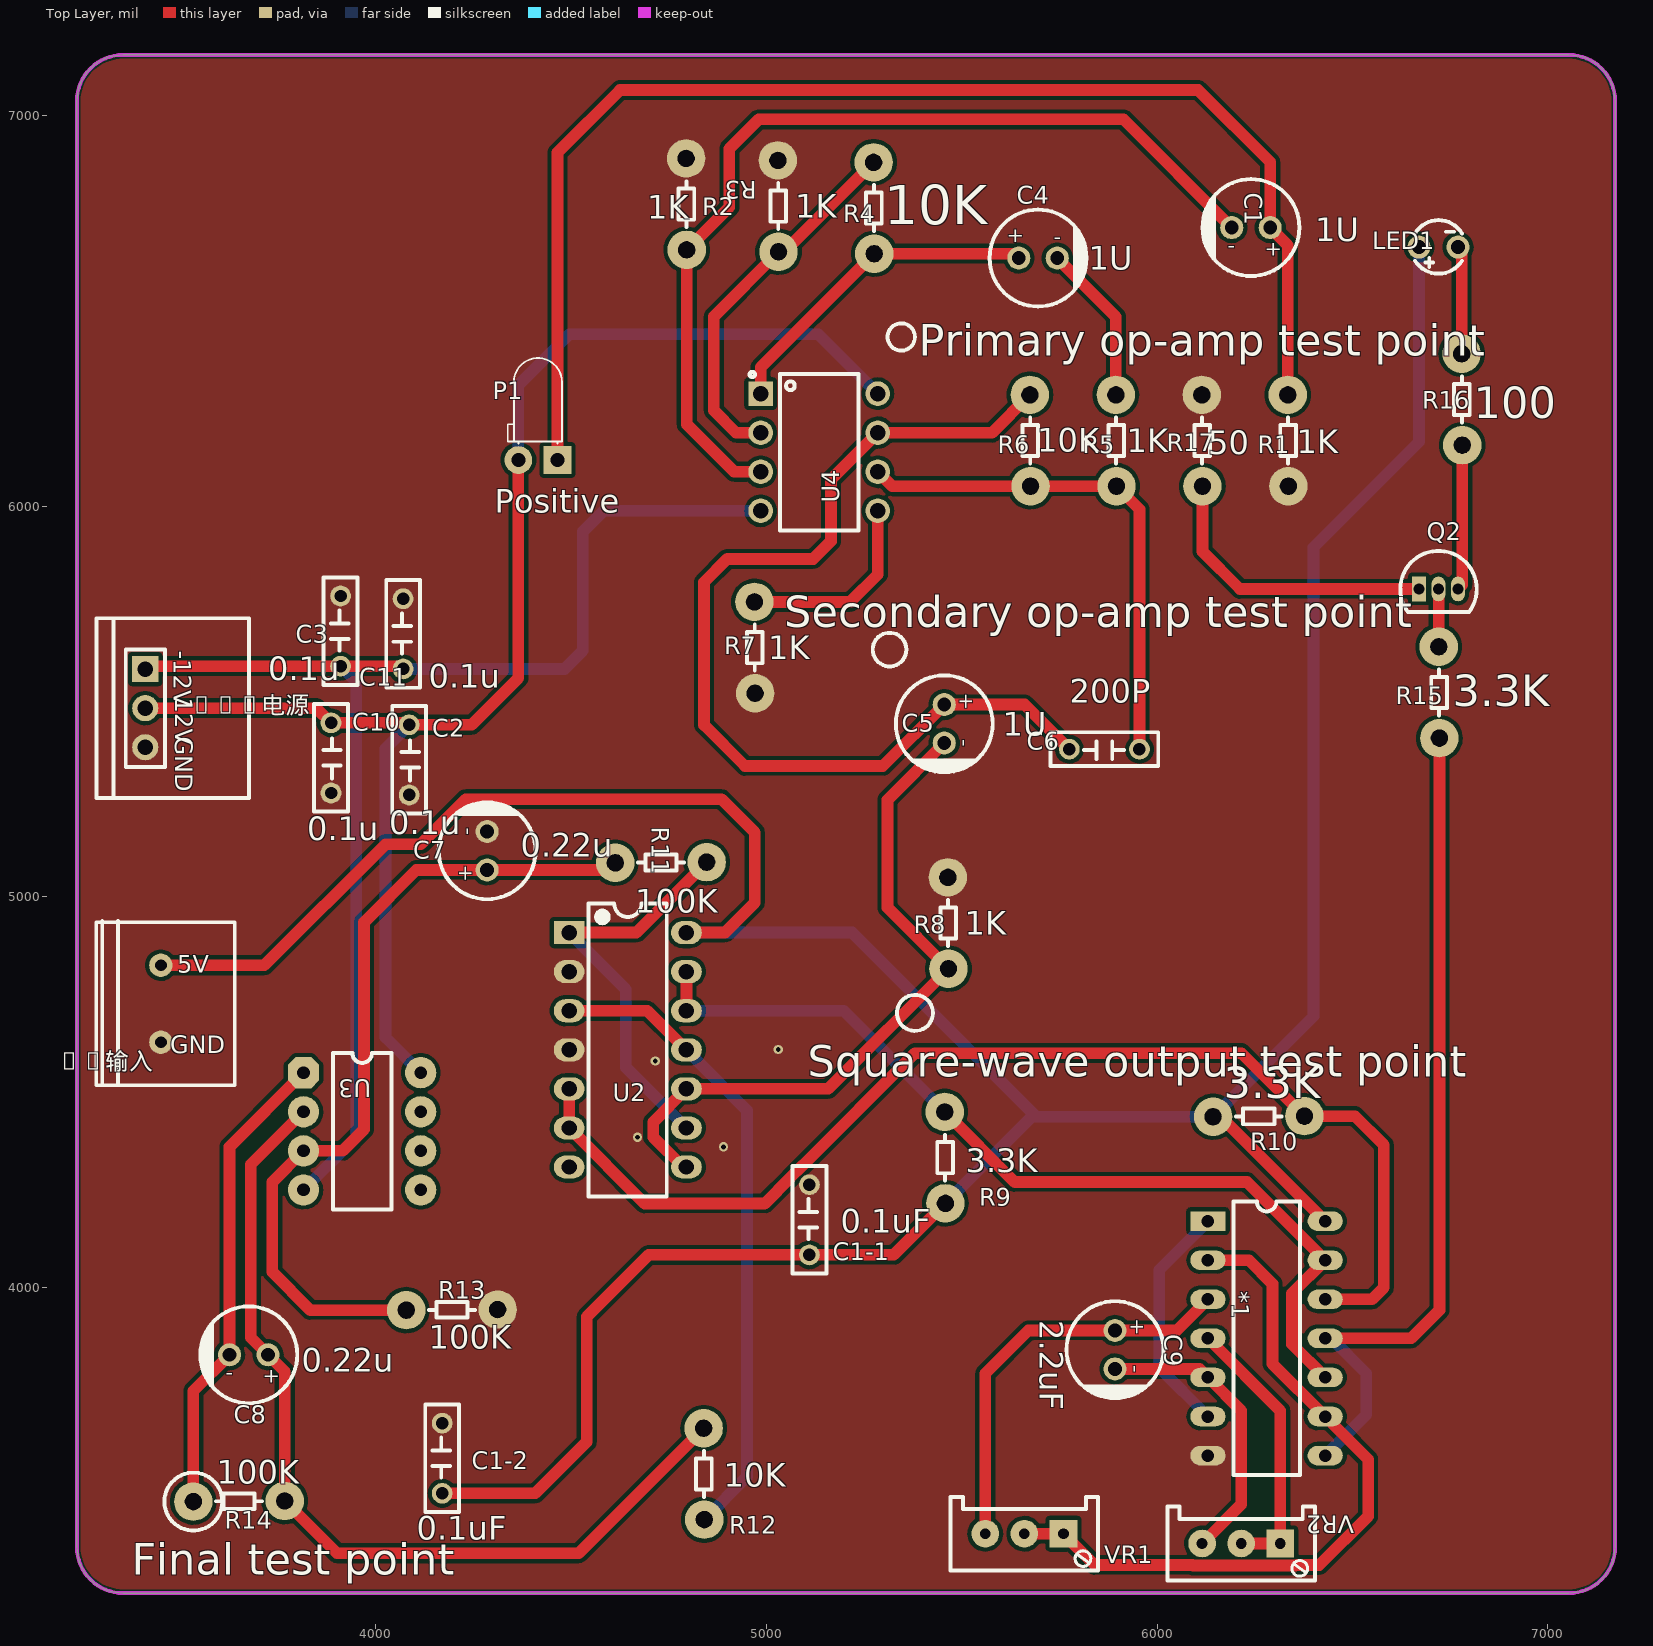
[diagram p0: Top Layer view]
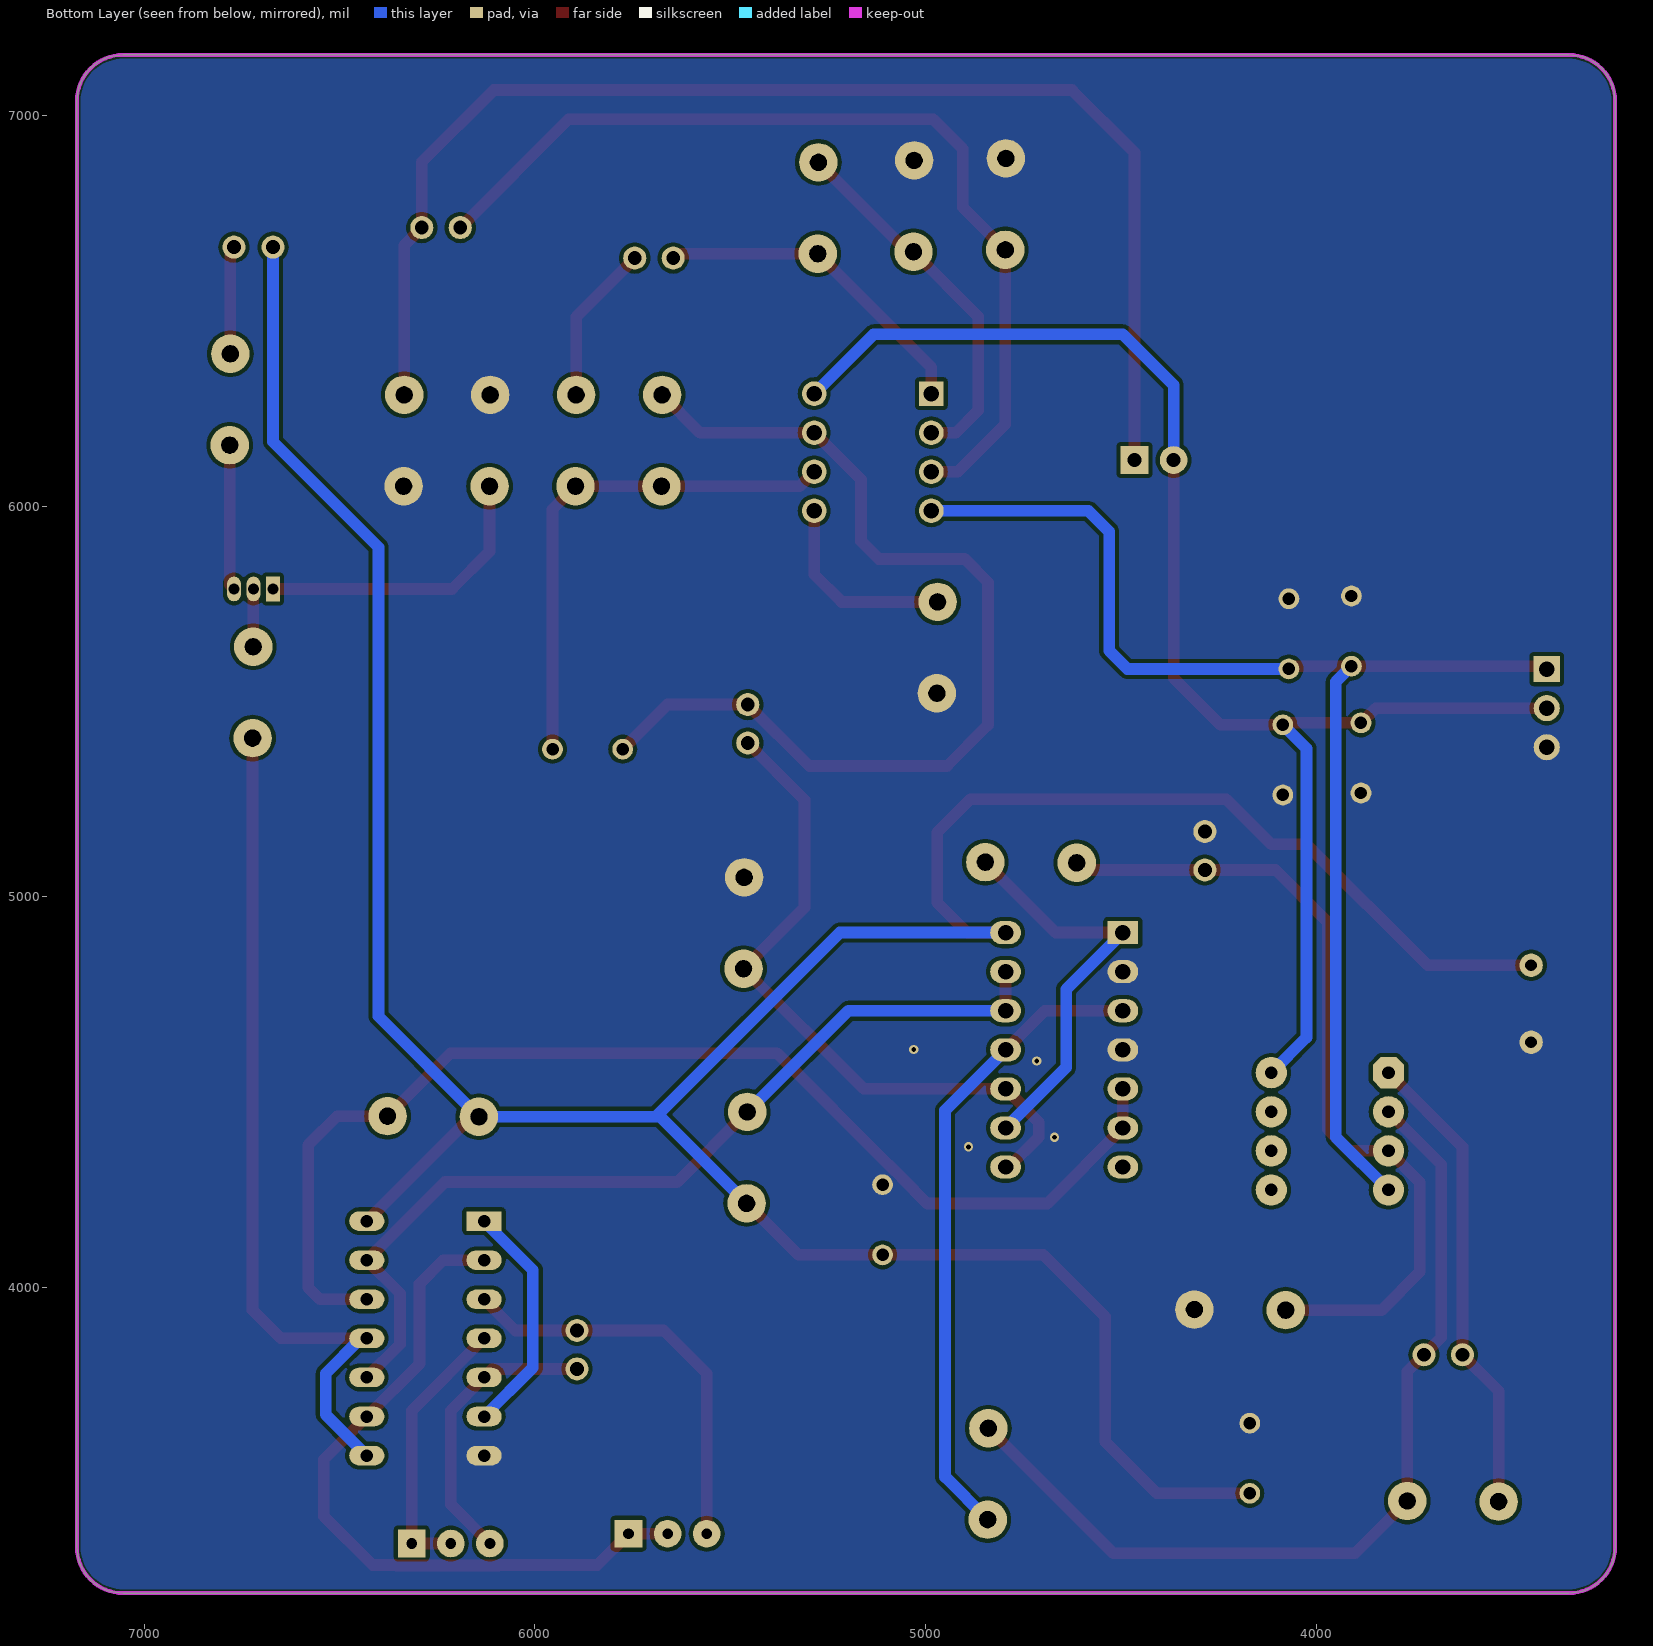
[diagram p1: Bottom Layer view, seen from below]
# Altium PCB MISC75397.pcbdoc
Units mil, origin at the board's own origin, x right, y up, seen from the top; angles counter-clockwise.
Board outline 3937.01 x 3937.01 mil, 2 copper layers (Top Layer, Bottom Layer), stack 62.206 mil thick; 41 components, 30 nets, 122 pads, 4 vias.

## Layer stack, top to bottom
Top Solder Mask Layer: solder mask 0.394, Dk 3.3
Top Layer: signal copper 1.379
Dielectric1: surface 59.449, FR4, Dk 4.5
Bottom Layer: signal copper 1.378
Bottom Solder Mask Layer: solder mask 0.394, Dk 3.3

## Board outline
3235,3336.1 ccw(c3353.11,3336.1) 3353.11,3217.99 7053.9,3217.99 ccw(c7053.9,3336.1) 7172.01,3336.1 7172.01,7036.89 ccw(c7053.9,7036.89) 7053.9,7155 3353.11,7155 ccw(c3353.11,7036.89) 3235,7036.89

## Design rules (kind name [scope] priority, off if disabled: settings)
BoardOutlineClearance copperThickness2oz_1 [All] p2 off: genericclearance=7.99 ignorepadtopadclearanceinfootprint=FALSE except(0: Arc-SplitContinuation Track-SplitContinuation SMDPad-SplitContinuation THPad-SplitContinuation Via-SplitContinuation Fill-SplitContinuation Region-SplitContinuation Poly-SplitContinuation Text-SplitContinuation Hole-SplitContinuation; 5.98: Arc-CutoutEdge Track-CutoutEdge SMDPad-CutoutEdge THPad-CutoutEdge Via-CutoutEdge Text-CutoutEdge; 6.89: Hole-OutlineEdge Hole-CutoutEdge; 10: Poly-OutlineEdge Poly-CutoutEdge; 11.81: Arc-OutlineEdge Track-OutlineEdge SMDPad-OutlineEdge THPad-OutlineEdge Via-OutlineEdge Fill-OutlineEdge Region-OutlineEdge Text-OutlineEdge Fill-CutoutEdge Region-CutoutEdge)
BoardOutlineClearance Plane_innerPlane_1 [All] p4 off: genericclearance=4.02 ignorepadtopadclearanceinfootprint=FALSE except(0: Arc-SplitContinuation Track-SplitContinuation SMDPad-SplitContinuation THPad-SplitContinuation Via-SplitContinuation Fill-SplitContinuation Region-SplitContinuation Poly-SplitContinuation Text-SplitContinuation Hole-SplitContinuation; 5.98: Arc-CutoutEdge Track-CutoutEdge SMDPad-CutoutEdge THPad-CutoutEdge Via-CutoutEdge Text-CutoutEdge; 6.89: Hole-OutlineEdge Hole-CutoutEdge; 10: Poly-OutlineEdge Poly-CutoutEdge; 11.81: Arc-OutlineEdge Track-OutlineEdge SMDPad-OutlineEdge THPad-OutlineEdge Via-OutlineEdge Fill-OutlineEdge Region-OutlineEdge Text-OutlineEdge Fill-CutoutEdge Region-CutoutEdge)
BoardOutlineClearance Copper_copperRegion_1 [All] p6 off: genericclearance=4.02 ignorepadtopadclearanceinfootprint=FALSE except(0: Arc-SplitContinuation Track-SplitContinuation SMDPad-SplitContinuation THPad-SplitContinuation Via-SplitContinuation Fill-SplitContinuation Region-SplitContinuation Poly-SplitContinuation Text-SplitContinuation Hole-SplitContinuation; 5.98: Arc-CutoutEdge Track-CutoutEdge SMDPad-CutoutEdge THPad-CutoutEdge Via-CutoutEdge Text-CutoutEdge; 6.89: Hole-OutlineEdge Hole-CutoutEdge; 10: Poly-OutlineEdge Poly-CutoutEdge; 11.81: Arc-OutlineEdge Track-OutlineEdge SMDPad-OutlineEdge THPad-OutlineEdge Via-OutlineEdge Fill-OutlineEdge Region-OutlineEdge Text-OutlineEdge Fill-CutoutEdge Region-CutoutEdge)
BoardOutlineClearance copperThickness1oz_1 [All] p8: genericclearance=4.02 ignorepadtopadclearanceinfootprint=FALSE except(0: Arc-SplitContinuation Track-SplitContinuation SMDPad-SplitContinuation THPad-SplitContinuation Via-SplitContinuation Fill-SplitContinuation Region-SplitContinuation Poly-SplitContinuation Text-SplitContinuation Hole-SplitContinuation; 5.98: Arc-CutoutEdge Track-CutoutEdge SMDPad-CutoutEdge THPad-CutoutEdge Via-CutoutEdge Text-CutoutEdge; 6.89: Hole-OutlineEdge Hole-CutoutEdge; 10: Poly-OutlineEdge Poly-CutoutEdge; 11.81: Arc-OutlineEdge Track-OutlineEdge SMDPad-OutlineEdge THPad-OutlineEdge Via-OutlineEdge Fill-OutlineEdge Region-OutlineEdge Text-OutlineEdge Fill-CutoutEdge Region-CutoutEdge)
Clearance copperThickness2oz [All] p1 off: gap=7.99 ignorepadtopadclearanceinfootprint=FALSE except(5.98: SMDPad-Track SMDPad-SMDPad THPad-Track SMDPad-THPad THPad-THPad Track-Via SMDPad-Via THPad-Via Via-Via Fill-SMDPad Region-SMDPad Fill-THPad Region-THPad Fill-Via Region-Via Fill-Fill Fill-Region Region-Region Arc-Track Arc-SMDPad Arc-THPad Arc-Via Fill-Arc Region-Arc Arc-Arc Text-Track SMDPad-Text Text-THPad Text-Via Fill-Text Region-Text Arc-Text Text-Text; 6.89: Hole-Track Hole-SMDPad Hole-THPad Hole-Via Fill-Hole Region-Hole Hole-Arc Hole-Text; 10: Poly-Track Poly-SMDPad Poly-THPad Poly-Via Poly-Fill Poly-Region Poly-Poly Poly-Arc Poly-Text Poly-Hole; 11.81: Fill-Track Region-Track)
Clearance Plane_innerPlane [All] p3 off: gap=4.02 ignorepadtopadclearanceinfootprint=FALSE except(5.98: SMDPad-Track SMDPad-SMDPad THPad-Track SMDPad-THPad THPad-THPad Track-Via SMDPad-Via THPad-Via Via-Via Fill-SMDPad Region-SMDPad Fill-THPad Region-THPad Fill-Via Region-Via Fill-Fill Fill-Region Region-Region Arc-Track Arc-SMDPad Arc-THPad Arc-Via Fill-Arc Region-Arc Arc-Arc Text-Track SMDPad-Text Text-THPad Text-Via Fill-Text Region-Text Arc-Text Text-Text; 6.89: Hole-Track Hole-SMDPad Hole-THPad Hole-Via Fill-Hole Region-Hole Hole-Arc Hole-Text; 10: Poly-Track Poly-SMDPad Poly-THPad Poly-Via Poly-Fill Poly-Region Poly-Poly Poly-Arc Poly-Text Poly-Hole; 11.81: Fill-Track Region-Track)
Clearance Copper_copperRegion [All] p5 off: gap=4.02 ignorepadtopadclearanceinfootprint=FALSE except(5.98: SMDPad-Track SMDPad-SMDPad THPad-Track SMDPad-THPad THPad-THPad Track-Via SMDPad-Via THPad-Via Via-Via Fill-SMDPad Region-SMDPad Fill-THPad Region-THPad Fill-Via Region-Via Fill-Fill Fill-Region Region-Region Arc-Track Arc-SMDPad Arc-THPad Arc-Via Fill-Arc Region-Arc Arc-Arc Text-Track SMDPad-Text Text-THPad Text-Via Fill-Text Region-Text Arc-Text Text-Text; 6.89: Hole-Track Hole-SMDPad Hole-THPad Hole-Via Fill-Hole Region-Hole Hole-Arc Hole-Text; 10: Poly-Track Poly-SMDPad Poly-THPad Poly-Via Poly-Fill Poly-Region Poly-Poly Poly-Arc Poly-Text Poly-Hole; 11.81: Fill-Track Region-Track)
Clearance copperThickness1oz [All] p7: gap=4.02 ignorepadtopadclearanceinfootprint=FALSE except(5.98: SMDPad-Track SMDPad-SMDPad THPad-Track SMDPad-THPad THPad-THPad Track-Via SMDPad-Via THPad-Via Via-Via Fill-SMDPad Region-SMDPad Fill-THPad Region-THPad Fill-Via Region-Via Fill-Fill Fill-Region Region-Region Arc-Track Arc-SMDPad Arc-THPad Arc-Via Fill-Arc Region-Arc Arc-Arc Text-Track SMDPad-Text Text-THPad Text-Via Fill-Text Region-Text Arc-Text Text-Text; 6.89: Hole-Track Hole-SMDPad Hole-THPad Hole-Via Fill-Hole Region-Hole Hole-Arc Hole-Text; 10: Poly-Track Poly-SMDPad Poly-THPad Poly-Via Poly-Fill Poly-Region Poly-Poly Poly-Arc Poly-Text Poly-Hole; 11.81: Fill-Track Region-Track)
DiffPairsRouting differentialPair [All] p1: maxlimit=6 minlimit=6 mostfreqgap=6 toplayer_minwidth=5 toplayer_prefwidth=10 toplayer_maxwidth=100 toplayer_mingap=6 toplayer_prefgap=6 toplayer_maxgap=6 bottomlayer_minwidth=5 bottomlayer_prefwidth=10 bottomlayer_maxwidth=100 bottomlayer_mingap=6 bottomlayer_prefgap=6 bottomlayer_maxgap=6 maxuncoupledlength=10
HoleToHoleClearance otherClearance [All] p1: gap=11.81 allowstackedmicrovias=TRUE
Length netLength [All] p1: minlimit=0 maxlimit=0
PasteMaskExpansion pasteMaskExpansion [All] p1: expansion=0
PlaneConnect innerPlane [All] p1: planeconnectstyle=Relief reliefexpansion=20 reliefentries=4 reliefconductorwidth=10 reliefairgap=10
PolygonConnect copperRegion [All] p1: connectstyle=Direct reliefconductorwidth=10 reliefentries=4 polygonreliefangle="90 Angle" airgapwidth=10 via.connectstyle=Relief via.reliefconductorwidth=10 via.reliefentries=4 via.polygonreliefangle="90 Angle" via.airgapwidth=10
RoutingVias viaSize [All] p1: holewidth=12.01 width=24.02 viastyle="Through Hole" minholewidth=11.81 minwidth=19.68 maxholewidth=248.03 maxwidth=393.7
SolderMaskExpansion solderMaskExpansion [IsVia] p1: expansion=-1000 istentingtop=TRUE
SolderMaskExpansion solderMaskExpansion [All] p2: expansion=2.01 istentingtop=FALSE
Width copperThickness2oz_2 [All] p1 off: maxlimit=100 minlimit=8 preferedwidth=10
Width copperThickness1oz_2 [All] p2: maxlimit=100 minlimit=5 preferedwidth=10

## Components (designator, comment, footprint, x,y, rotation, side; value= is the part's Value field where it differs from the comment)
5V输入 "5V output" 2INT 3450,4627.99 r90 top
12V电源 "3PIN" 3PIN 3410,5482.99 r90 top
*1 "74HC04" DIP14 6130,4170 r0 top
C1 "220uF" CAP-TH_BD6.3-P2.50-D0.5-FD 6240,6712.99 r180 top
C1-1 "" 电容直插 5109.86,4173.33 r270 top
C1-2 "" 电容直插 4170,3562.99 r270 top
C2 "" 电容直插 4085.44,5350.79 r90 top
C3 "" 电容直插 3910,5680 r270 top
C4 "220uF" CAP-TH_BD6.3-P2.50-D0.5-FD 5695,6635 r0 top
C5 "220uF" CAP-TH_BD6.3-P2.50-D0.5-FD 5455,5442.99 r270 top
C6 "" 电容直插 5865,5377.99 r0 top
C7 "220uF" CAP-TH_BD6.3-P2.50-D0.5-FD 4285,5117.99 r90 top
C8 "220uF" CAP-TH_BD6.3-P2.50-D0.5-FD 3675,3827.99 r180 top
C9 "220uF" CAP-TH_BD6.3-P2.50-D0.5-FD 5891.99,3841.01 r270 top
C10 "" 电容直插 3885.44,5355.79 r90 top
C11 "" 电容直插 4070,5672.99 r270 top
LED1 "3A4GUD" LED-TH_BD3.5-P2.54-RD-GREEN 6720,6662.99 r180 top
P1 "" LED_D3.0mm_Horizontal_O1.27mm_Z2.0mm 4415,6117.99 r180 top
Q2 "S9018" TO-92-3_L4.9-W3.7-P1.27-L 6720,5787.99 r0 top
R1 "" D45-V(直插) 6335,6167.99 r270 top
R2 "" D45-V(直插) 4795,6772.99 r90 top
R3 "" D45-V(直插) 5030,6767.99 r90 top
R4 "" D45-V(直插) 5275,6762.99 r90 top
R5 "" D45-V(直插) 5895,6167.99 r90 top
R6 "" D45-V(直插) 5675,6167.99 r90 top
R7 "" D45-V(直插) 4970,5637.99 r90 top
R8 "" D45-V(直插) 5465,4932.99 r90 top
R9 "" D45-V(直插) 5457.07,4332.55 r270 top
R10 "" D45-V(直插) 6260.01,4438 r180 top
R11 "" D45-V(直插) 4730,5087.99 r180 top
R12 "" D45-V(直插) 4840,3522.99 r90 top
R13 "" D45-V(直插) 4195,3942.99 r0 top
R14 "" D45-V(直插) 3650,3452.99 r180 top
R15 "" D45-V(直插) 6721.47,5523.22 r90 top
R16 "" D45-V(直插) 6780,6272.99 r90 top
R17 "" D45-V(直插) 6115,6167.99 r270 top
U2 "CD4066DN" PDIP-14_L19.3-W6.5-P2.54-LS7.6-BL 4645,4608.54 r270 top
U3 "LF353" DIP-8 3815,4550 r0 top
U4 "" DIP-8_L9.9-W6.4-P2.54-LS7.6-BL 5135,6137.99 r270 top
VR1 "101" 3296W 5660,3370 r180 top
VR2 "101" 3296W 6215,3345 r180 top

## Footprints (in the part's own frame and the unit in brackets; to place one, negate y for a bottom-side part, rotate by r counter-clockwise, add the part's x,y. Pads: shape width x height; smd on the part's side, far side on the other; paste and mask are expansions set on the pad)
2INT [mil]
  round 60 hole 30: 1(196.85,0) 2(0,0)
  silkscreen extent -110,-189 310,165
3PIN [mm]
  rect 1.7x1.7 hole 1: 1(2.54,0)
  round 1.7 hole 1: 2(0,0) 3(-2.54,0)
  silkscreen extent -3.84,-1.27 3.81,1.27
3296W [mm]
  rect 1.8x1.8 hole 0.7: 1(-2.54,0)
  round 1.8 hole 0.7: 2(0,0) 3(2.54,0)
  silkscreen extent -4.8,-2.4 4.8,2.4
CAP-TH_BD6.3-P2.50-D0.5-FD [mm]
  round 1.5 hole 0.9 paste+0 mask+0.05: 1(-1.25,0) 2(1.25,0)
  silkscreen extent -3.15,-3.15 3.21,3.15
D45-V(直插) [mm]
  round 2.5 hole 1.1 slot 1.105 at 90 deg: 1(-2.97,-0.02) 2(2.97,0.02)
  silkscreen extent -1.49,-0.51 1.49,0.51
DIP14 [mil]
  rect 90x50 hole 32: 1(0,0)
  oval 90x50 hole 32: 2(0,-100) 3(0,-200) 4(0,-300) 5(0,-400) 6(0,-500) 7(0,-600) 8(300,-600) 9(300,-500) 10(300,-400) 11(300,-300) 12(300,-200) 13(300,-100) 14(300,0)
  silkscreen extent 65,-650 235,50
DIP-8 [mil]
  oct 80x80 hole 32: 1(0,0)
  round 80 / inner round 50 / far side round 80 hole 32: 2(0,-100) 3(0,-200) 4(0,-300) 5(300,-300) 6(300,-200) 7(300,-100) 8(300,0)
  silkscreen extent 75,-350 225,50
DIP-8_L9.9-W6.4-P2.54-LS7.6-BL [mil]
  rect 63x63 hole 39.37: 1(-150,-150)
  round 63 hole 39.37: 2(-50,-150) 3(50,-150) 4(150,-150) 5(150,150) 6(50,150) 7(-50,150) 8(-150,150)
  silkscreen extent -206,-178 200,100
LED-TH_BD3.5-P2.54-RD-GREEN [mm]
  round 1.5 hole 0.9: 1(-1.27,0) 2(1.27,0)
  silkscreen extent -1.52,-1.75 1.52,1.73
LED_D3.0mm_Horizontal_O1.27mm_Z2.0mm [mm]
  rect 1.8x1.8 hole 0.9 paste+0 mask+0: 1(-1.27,0)
  round 1.8 hole 0.9 paste+0 mask+0: 2(1.27,0)
  silkscreen extent -1.56,-6.63 1.96,-1.08
PDIP-14_L19.3-W6.5-P2.54-LS7.6-BL [mm]
  rect 1.5x2 hole 1: 1(-7.62,-3.81)
  oval 1.5x2 hole 1: 2(-5.08,-3.81) 3(-2.54,-3.81) 4(0,-3.81) 5(2.54,-3.81) 6(5.08,-3.81) 7(7.62,-3.81) 8(7.62,3.81) 9(5.08,3.81) 10(2.54,3.81) 11(0,3.81) 12(-2.54,3.81) 13(-5.08,3.81) 14(-7.62,3.81)
  silkscreen extent -9.53,-2.55 9.53,2.53
TO-92-3_L4.9-W3.7-P1.27-L [mm]
  rect 0.9x1.6 hole 0.7: 1(-1.27,0)
  oval 0.9x1.6 hole 0.7: 2(0,0) 3(1.27,0)
  silkscreen extent -2.48,-1.5 2.48,2.48
电容直插 [mm]
  round 1.35 hole 0.81: 1(-2.286,0) 2(2.276,0)
  silkscreen extent -3.5,-1.1 3.5,1.1

## Via types
v1: diameter 24.02, hole 12, Top Layer to Bottom Layer, 4 vias

## Nets (pads, with @x,y where several pads share a name; then routed paths per layer and width w, separated by ;. In a path a pad name is that pad's centre, name@x,y a point inside that pad or via, vN(x,y) a via of type N, cw(c..) or ccw(c..) an arc to the next point about the centre after c; other vN are vias at no path point)
1: C4.1 R4.1 U4.1 | length 853.1
  Top Layer w30: U4.1 4985,6355.27 R4.1 5634.73,6646.06 C4.1
2: R3.1 R4.2 U4.2 | length 956.6
  Top Layer w30: U4.2 4922.01,6187.99 4865,6245 4865,6485.28 R3.1 5045.35,6651.06 R4.2
3: C1.2 R2.1 U4.3 | length 2422
  Top Layer w30: U4.3 4917.01,6087.99 4795.78,6209.22 R2.1 4905,6765.28 4905,6915 4980,6990 5913.78,6990 C1.2
5: R7.2 U4.5 | length 507.8
  Top Layer w30: R7.2 5214.92,5754.92 5285,5825 U4.5
6: C6.2 R5.1 R6.1 U4.6 | length 1323.5
  Top Layer w30: U4.6 5321.92,6051.06 R6.1 R5.1 5954.62,5992.23 C6.2
7: C5.1 C6.1 R6.2 U4.7 | length 2581.5
  Top Layer w30: R6.2 5577.28,6187.99 U4.7 5165,6067.99 5165,5910 5120,5865 4900,5865 4840,5805 4840,5440 4945,5335 5297.8,5335 C5.1 5660.79,5492.2 C6.1
12V: 12V电源.2 C2.2 C10.2 P1.2 U3.8 U4.8 | length 3761.7
  Top Layer w30: 12V电源.2 3847.86,5482.99 C10.2 4080.44,5445.41 C2.2 4245.41,5440.41 4365,5560 P1.2
  Bottom Layer w30: C2.2 4025,5379.96 4025,4640 U3.8 ; P1.2 4365,6310 4495,6440 5132.98,6440 U4.8
$1N1572: C1.1 P1.1 R1.1 | length 3368.3
  Top Layer w30: P1.1 4465,6905 4625,7065 6105,7065 6289.21,6880.79 C1.1 6334.22,6667.99 R1.1
$1N2846: C4.2 R5.2 | length 412.2
  Top Layer w30: C4.2 5894.22,6484.99 R5.2
$1N2910: C5.2 R8.1 U2.8 U2.10 | length 1775.9
  Top Layer w30: U2.8 4786.46,4308.54 4710,4385 4710,4423.54 U2.10 5158.26,4508.54 R8.1 5310,4971.85 5310,5248.78 C5.2
$1N2968: R11.1 U2.1 U2.9 | length 1050.9
  Top Layer w30: U2.1 4666.69,4908.54 R11.1
  Bottom Layer w30: U2.1 4640,4763.54 4640,4563.54 U2.9
$1N3169: R12.1 U2.3 U2.11 | length 1653.3
  Top Layer w30: U2.3 4695,4708.54 U2.11
  Bottom Layer w30: U2.11 4950,4453.54 4950,3515.28 R12.1
$1N3229: C8.1 R12.2 R14.1 U3.2 | length 2348.4
  Top Layer w30: U3.2 3680,4315 3680,3872.2 C8.1 3766.93,3785.27 R14.1 3900.71,3320 4519.29,3320 R12.2
$1N3233: C7.1 R11.2 R13.1 U3.3 | length 2140.6
  Top Layer w30: R13.1 3832.79,3942.21 3735,4040 3735,4270 U3.3 3915,4350 3970,4405 3970,4935 4103.78,5068.78 C7.1 4594.65,5068.78 R11.2
$1N3822: *1.12 R10.1 U2.5 U2.6 | length 3049.8
  Top Layer w30: U2.5 U2.6 4688.54,4215 4995,4215 5062.3,4282.3 5062.3,4283.03 5090.16,4310.89 5090.89,4310.89 5380,4600 6215.72,4600 R10.1 6506.22,4438.78 6580,4365 6580,4000 6550,3970 *1.12
$1N4613: *1.10 *1.13 R9.1 U2.12 U2.13 | length 2369.9
  Top Layer w30: U2.12 U2.13 ; R9.1 5635.77,4270 6230,4270 *1.13 6345,3985 6345,3855 *1.10
  Bottom Layer w30: U2.12 5197.23,4708.54 R9.1
$1N4655: *1.8 *1.11 R15.1 | length 2182
  Top Layer w30: *1.11 6650,3870 6722.26,3942.26 R15.1
  Bottom Layer w30: *1.8 6535,3675 6535,3780 6445,3870 *1.11
$1N4661: *1.1 *1.6 | length 603.6
  Bottom Layer w30: *1.6 6005,3795 6005,4045 *1.1
$1N4668: *1.2 *1.9 VR1.1 VR1.2 | length 1852
  Top Layer w30: VR1.2 VR1.1 5840,3290 6090.21,3290 6091.63,3288.58 6350.43,3288.58 ccw(c6350.43,3309.57) 6358.01,3290 6415,3290 6540,3415 6540,3560 *1.9 6295,3805 6295,4010 6235,4070 *1.2
$1N4723: *1.3 C9.1 VR1.3 | length 1058.7
  Top Layer w30: VR1.3 5560,3780 5670.22,3890.22 C9.1 6050.22,3890.22 *1.3
$1N4812: *1.5 C9.2 VR2.3 | length 748.7
  Top Layer w30: C9.2 6108.2,3791.8 *1.5 6215,3685 6215,3445 VR2.3
$1N4856: *1.4 VR2.1 VR2.2 | length 701.6
  Top Layer w30: *1.4 6315,3685 VR2.1 VR2.2
$1N5161: LED1.1 R16.2 | length 276.9
  Top Layer w30: LED1.1 6779.22,6653.78 R16.2
$1N5332: Q2.2 R15.2 | length 148.1
  Top Layer w30: Q2.2 6720.69,5787.3 R15.2
$1N5334: Q2.3 R16.1 | length 372.5
  Top Layer w30: Q2.3 6780.78,5798.78 R16.1
$1N5336: Q2.1 R17.2 | length 760.9
  Top Layer w30: R17.2 6115.78,5884.22 6212.01,5787.99 Q2.1
+5V: 5V输入.1 *1.14 C1-1.2 C1-2.2 LED1.2 R9.2 R10.2 U2.14 | length 8610.5
  Top Layer w30: 5V输入.1 3714.84,4824.84 4025,5135 4115,5135 4230,5250 4885,5250 4970,5165 4970,4985 4893.54,4908.54 U2.14 ; C1-2.2 4408.37,3473.37 4540,3605 4540,3925 4698.71,4083.71 C1-1.2 5325.95,4083.71 R9.2 ; R10.2 6162.79,4437.21 *1.14
  Bottom Layer w30: U2.14 5219.58,4908.54 5690.91,4437.21 ; R9.2 5679.45,4437.21 5690.91,4437.21 ; LED1.2 6670,6165 6400,5895 6400,4694.14 R10.2 5690.91,4437.21
-12V: 12V电源.1 C3.2 C11.2 U3.4 U4.4 | length 3340.1
  Top Layer w30: 12V电源.1 3417.39,5590.38 C3.2 4062.99,5590.38 C11.2
  Bottom Layer w30: U3.4 3950,4385 3950,5550.38 C3.2 ; C11.2 4483.37,5583.37 4530,5630 4530,5935 4582.99,5987.99 U4.4
GND: 5V输入.2 12V电源.3 *1.7 C1-1.1 C1-2.1 C2.1 C3.1 C7.2 C10.1 C11.1 R1.2 R2.2 R3.2 R7.1 R8.2 R13.2 R17.1 U2.2 U2.4
  other v1: 4890,4360 4670,4385 4715,4580 5030.14,4609.27
OUT: C8.2 R14.2 U3.1 | length 1214.6
  Top Layer w30: R14.2 3533.07,3735.27 C8.2 3625.79,4360.79 U3.1
pads on no net: U2.7 U3.5 U3.6 U3.7

## Polygon pours and split planes (outlines as drawn)
GND on Top Layer (solid, remove dead copper, pour order 0): 3015,7405 3015,3000 7360,3000 7360,7405
GND on Bottom Layer (solid, remove dead copper, pour order 2): 3000,7520 3000,3010 7725,3010 7725,7520

## Keep-outs
Board Outline Layer:
  the board outline again, w10

## Silkscreen, mask and mechanical layers (free items; w line width, h text height)
Top Silkscreen Layer:
  circle w10: c5345,6432.99 r35
  circle w10: c5315,5632.99 r43.01
  circle w10: c5380,4702.99 r46.1
  circle w10: c3533.07,3452.21 r74.1
  lines w10: 3328.4,5252.99 3328.4,5712.99 ; 3285,5252.99 3675,5252.99 3675,5712.99 3285,5712.99 3285,5252.99
  text "1K" at 5073.55,6737.99 h60
  text "1K" at 4695,6735 h60
  text "10K" at 5301.7,6721.29 h100
  text "1U" at 6404.59,6677.89 h60
  text "1U" at 5825,6605 h60
  text "Primary op-amp test point" at 5390,6385 h80
  text "100" at 6810,6225 h80
  text "10K" at 5693.35,6139.64 h60
  text "1K" at 5922.65,6137.99 h60
  text "1K" at 6357.65,6135.34 h60
  text "50" at 6130.3,6132.69 h60
  text "Positive" at 4305,5982.99 h60
  text "Secondary op-amp test point" at 5045,5690 h80
  text "-12V" at 3482.5,5630.49 h45 r270
  text "1K" at 5004.13,5607.99 h60
  text "0.1u" at 3725,5555 h60
  text "0.1u" at 4135,5535 h60
  text "12V" at 3486.25,5509.24 h45 r270
  text "200P" at 5776.7,5496.29 h60
  text "3.3K" at 6756.82,5488.22 h80
  text "1U" at 5604.43,5412.99 h60
  text "GND" at 3486.25,5409.24 h45 r270
  text "0.1u" at 4035,5160 h60
  text "0.1u" at 3825,5145 h60
  text "0.22u" at 4370.86,5102.44 h60
  text "100K" at 4664.05,4959.5 h60
  text "1K" at 5507.87,4902.99 h60
  text "5V" at 3492.5,4805.49 h45
  text "GND" at 3473.75,4599.24 h45
  text "Square-wave output test point" at 5105,4540 h80
  text "3.3K" at 6170,4485 h80
  text "3.3K" at 5510,4295 h60
  text "0.1uF" at 5190,4140 h60
  text "2.2uF" at 5698.99,3916.01 h60 r270
  text "100K" at 4135,3842.99 h60
  text "0.22u" at 3810,3785 h60
  text "100K" at 3593.1,3497.99 h60
  text "10K" at 4890,3490 h60
  text "0.1uF" at 4105,3355 h60
  text "Final test point" at 3375,3265 h80